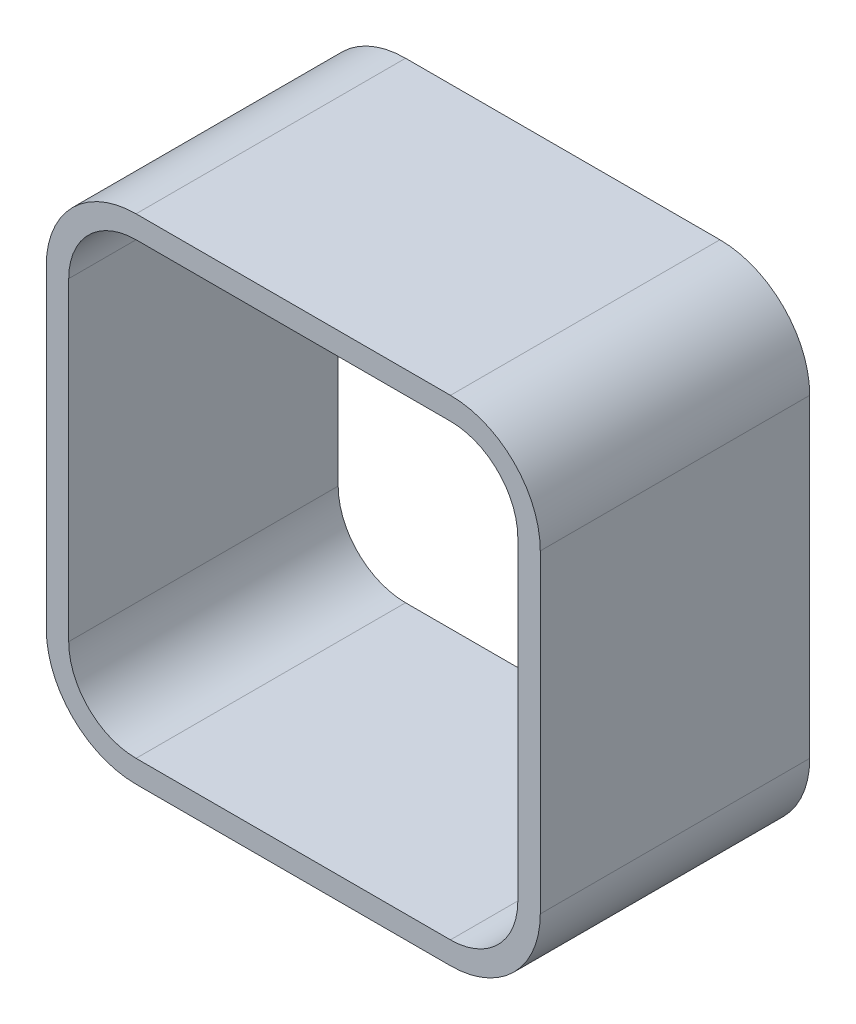
from build123d import *

# Parameters (mm, degrees)
EXTRUDE_1_DEPTH = 120


with BuildPart() as part:
    # 草图1 → 凸台-拉伸1 (new body)
    with BuildSketch(Plane.XY):
        with BuildLine():
            Line((-70, 110), (70, 110))
            ThreePointArc((70, 110), (98.284271247, 98.284271247), (110, 70))
            Line((110, 70), (110, -70))
            ThreePointArc((110, -70), (98.284271247, -98.284271247), (70, -110))
            Line((70, -110), (-70, -110))
            ThreePointArc((-70, -110), (-98.284271247, -98.284271247), (-110, -70))
            Line((-110, -70), (-110, 70))
            ThreePointArc((-110, 70), (-98.284271247, 98.284271247), (-70, 110))
        make_face()
        with BuildLine():
            Line((-70, 100), (70, 100))
            ThreePointArc((70, 100), (91.213203436, 91.213203436), (100, 70))
            Line((100, 70), (100, -70))
            ThreePointArc((100, -70), (91.213203436, -91.213203436), (70, -100))
            Line((70, -100), (-70, -100))
            ThreePointArc((-70, -100), (-91.213203436, -91.213203436), (-100, -70))
            Line((-100, -70), (-100, 70))
            ThreePointArc((-100, 70), (-91.213203436, 91.213203436), (-70, 100))
        make_face(mode=Mode.SUBTRACT)
    extrude(amount=EXTRUDE_1_DEPTH)


solid = part.part
